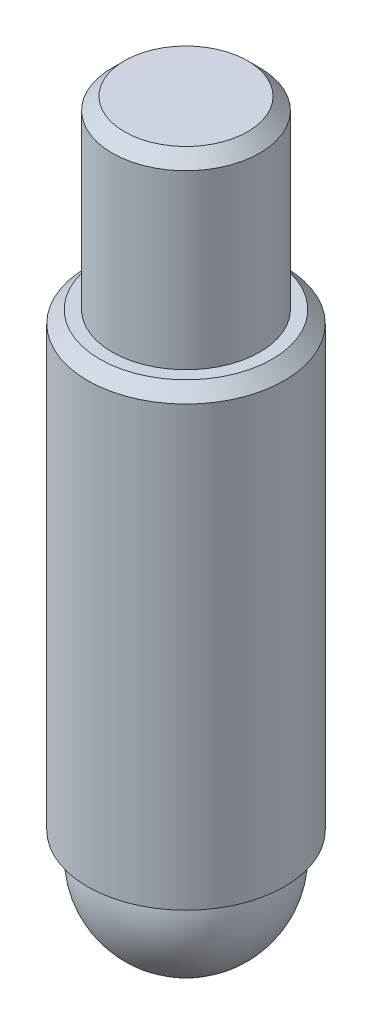
SolidWorks part; units mm, degrees
ref_plane "Front Plane" through (0, 0, 0) normal (0, 0, 1) x (1, 0, 0)
ref_plane "Top Plane" through (0, 0, 0) normal (0, 1, 0) x (1, 0, 0)
ref_plane "Right Plane" through (0, 0, 0) normal (1, 0, 0) x (0, 0, -1)
other "Configuration Table"
sketch "Sketch1" plane through (0, 0, 0) normal (0, 0, 1) x (1, 0, 0)
  line L0 (0, 0) -> (0, 30) construction
  line L1 (-2, 0) -> (-2, 27)
  line L2 (-4, 30) -> (-8, 30)
  line L3 (-8, 30) -> (-8, 8.3924)
  line L5 (-2, 0) -> (-2.5, 0)
  line L6 (-8, 8.3924) -> (-6.75, 8.3924)
  line L7 (-4, 30) -> (-4, 27)
  line L8 (-4, 27) -> (-2, 27)
  arc A2 (-6.75, 8.3924) -> (-2.5, 0) centre (0, 6.5383) ccw
  dimension "D6" = 3
  dimension "D7" = 14
  dimension "D1" = 8
  dimension "D2" = 2
  dimension "D3" = 4
  dimension "D4" = 30
  dimension "D5" = 0.5
  dimension "D8" = 1.25
revolve "Revolve2" add sketch "Sketch1" angle 360 about L0
sketch "Sketch2" plane through (0, 30, 0) normal (0, 1, 0) x (1, 0, 0)
  line L2 (-4, 6.9282) -> (-4, 4.4721)
  line L3 (4, 4.4721) -> (4, 6.9282)
  arc A1 (-4, 6.9282) -> (4, 6.9282) centre (0, 0) ccw
  circle A2 centre (0, 0) radius 2 construction
  arc A4 (-4, 4.4721) -> (4, 4.4721) centre (0, 0) ccw
  dimension "D1" = 4
  dimension "D3" = 6
  dimension "D2" = 4
extrude "Boss-Extrude1" add sketch "Sketch2" along normal blind 10
sketch "Sketch3" plane through (0, 40, 0) normal (0, 1, 0) x (1, 0, 0)
  circle A0 centre (0, 0) radius 8
  dimension "D1" = 16
extrude "Boss-Extrude2" add sketch "Sketch3" along normal blind 5
sketch "Sketch4" plane through (0, 45, 0) normal (0, 1, 0) x (1, 0, 0)
  circle A0 centre (0, 0) radius 6
  dimension "D1" = 12
extrude "Boss-Extrude3" add sketch "Sketch4" along normal blind 15
cosmetic thread "Cosmetic Thread1" parameters "D2"=11
chamfer "Chamfer1" distance 1 angle 45 2 edges at (0, 60, 6) (0, 45, 8)
